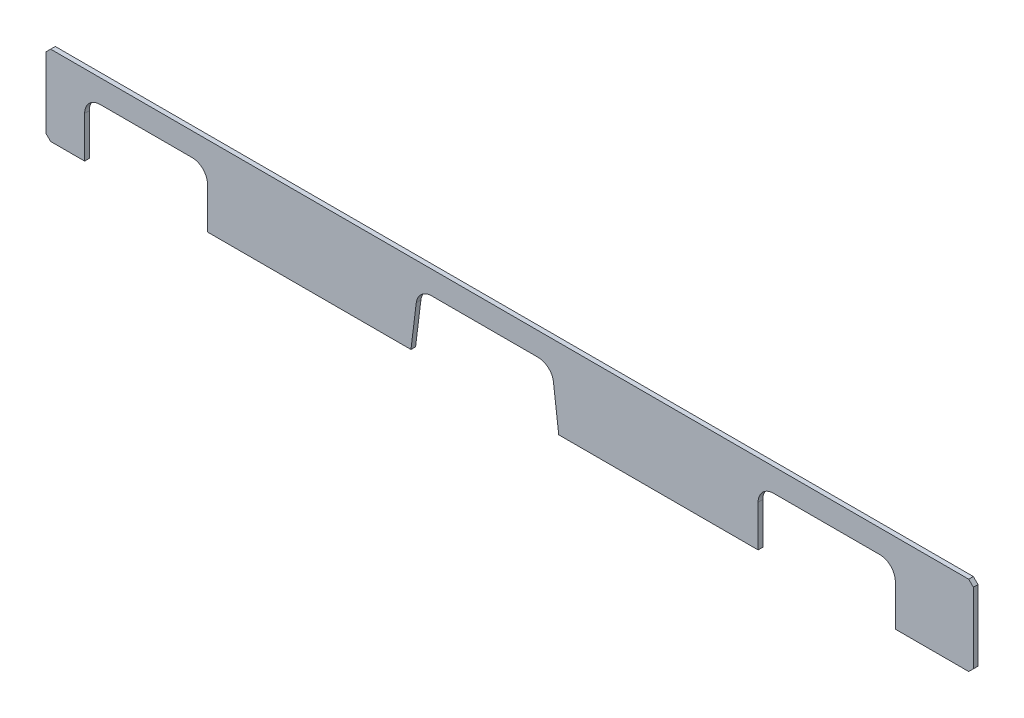
SolidWorks part; units mm, degrees
ref_plane "Front Plane" through (0, 0, 0) normal (0, 0, 1) x (1, 0, 0)
ref_plane "Top Plane" through (0, 0, 0) normal (0, 1, 0) x (1, 0, 0)
ref_plane "Right Plane" through (0, 0, 0) normal (1, 0, 0) x (0, 0, -1)
sketch "Sketch1" plane through (0, 0, 0) normal (0, 0, 1) x (1, 0, 0)
  line L0 (140, 147) -> (378, 147)
  line L1 (12, 0) -> (100, 0)
  line L2 (0, 12) -> (0, 195)
  line L3 (12, 207) -> (2388, 207)
  line L4 (2400, 12) -> (2400, 195)
  line L5 (100, 107) -> (100, 0)
  line L6 (418, 107) -> (418, 0)
  line L7 (944.5, 419.3573) -> (944.5, -282.3915) construction
  line L8 (1327, 419.3573) -> (1327, -227.6679) construction
  line L9 (1843, 107) -> (1843, 0)
  line L10 (2198, 107) -> (2198, 0)
  line L11 (944.5, 0) -> (958.2365, 111.8748)
  line L12 (1327, 0) -> (1313.2635, 111.8748)
  line L13 (0, 195) -> (12, 207)
  line L14 (2400, 195) -> (2388, 207)
  line L15 (997.9383, 147) -> (1273.5617, 147)
  line L16 (1883, 147) -> (2158, 147)
  line L17 (0, 12) -> (12, 0)
  line L18 (2388, 0) -> (2400, 12)
  line L19 (2198, 0) -> (2388, 0)
  line L20 (1327, 0) -> (1843, 0)
  line L21 (418, 0) -> (944.5, 0)
  arc A0 (2198, 107) -> (2158, 147) centre (2158, 107) ccw
  arc A1 (1843, 107) -> (1883, 147) centre (1883, 107) cw
  arc A2 (1313.2635, 111.8748) -> (1273.5617, 147) centre (1273.5617, 107) ccw
  arc A3 (958.2365, 111.8748) -> (997.9383, 147) centre (997.9383, 107) cw
  arc A4 (418, 107) -> (378, 147) centre (378, 107) ccw
  arc A5 (100, 107) -> (140, 147) centre (140, 107) cw
  point P0 (0, 0)
  point P1 (2400, 207)
  point P2 (0, 207)
  point P3 (2400, 0)
  dimension "D16" = 40
  dimension "D17" = 40
  dimension "D18" = 40
  dimension "D19" = 40
  dimension "D20" = 40
  dimension "D21" = 40
  dimension "D1" = 2400
  dimension "D2" = 207
  dimension "D3" = 60
  dimension "D4" = 100
  dimension "D5" = 318
  dimension "D6" = 202
  dimension "D7" = 355
  dimension "D8" = 526.5
  dimension "D9" = 382.5
  dimension "D10" = 83
  dimension "D11" = 83
  dimension "D12" = 12
  dimension "D13" = 45
  dimension "D14" = 12
  dimension "D15" = 45
  dimension "D22" = 12
  dimension "D23" = 45
  dimension "D24" = 12
  dimension "D25" = 45
extrude "Boss-Extrude1" add sketch "Sketch1" along normal blind 12
